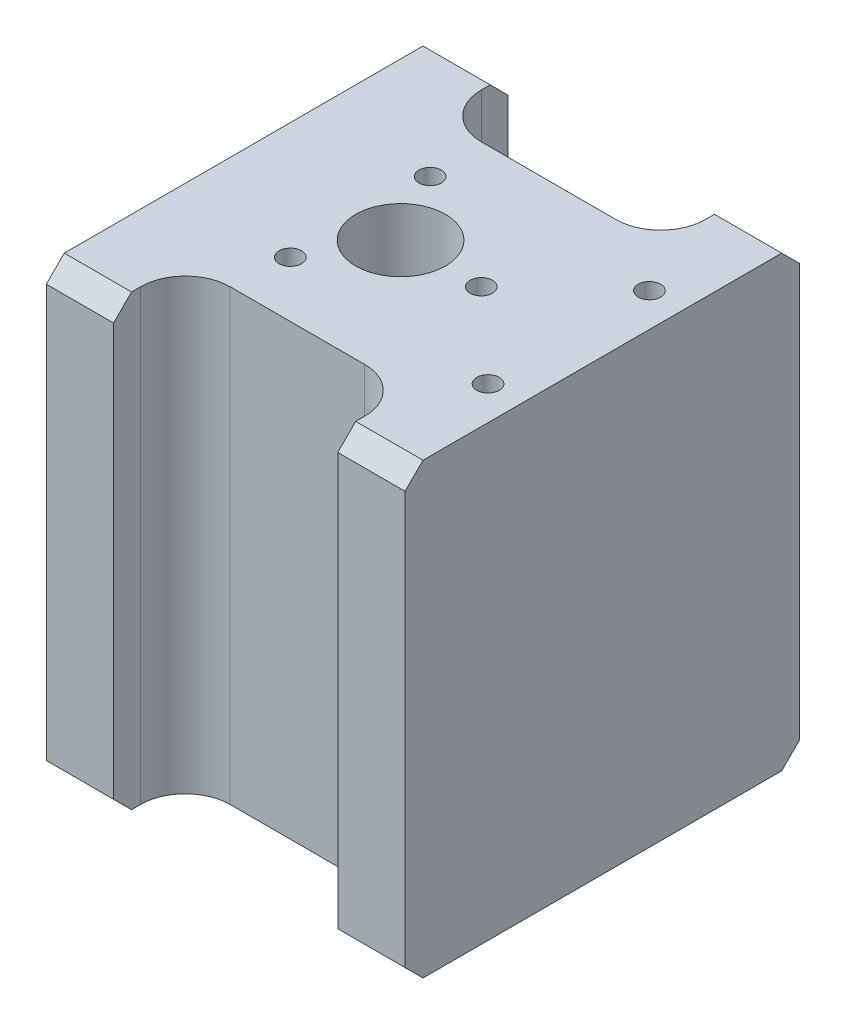
SolidWorks part; units mm, degrees
material "A6061"
ref_plane "Front Plane" through (0, 0, 0) normal (0, 0, 1) x (1, 0, 0)
ref_plane "Top Plane" through (0, 0, 0) normal (0, 1, 0) x (1, 0, 0)
ref_plane "Right Plane" through (0, 0, 0) normal (1, 0, 0) x (0, 0, -1)
sketch "Sketch1" plane through (0, 0, 0) normal (0, 0, 1) x (1, 0, 0)
  line L1 (-20, 25) -> (20, 25)
  line L2 (-20, 25) -> (-20, -25)
  line L3 (-20, -25) -> (20, -25)
  line L4 (20, 25) -> (20, -25)
  line L5 (-20, 25) -> (20, -25) construction
  line L6 (-20, -25) -> (20, 25) construction
  point P0 (0, 0)
  dimension "D1" = 40
  dimension "D2" = 50
extrude "Boss-Extrude1" add sketch "Sketch1" along normal blind 44
sketch "Sketch2" plane through (0, 25, 0) normal (0, 1, 0) x (1, 0, 0)
  line L0 (-20, -22) -> (20, -22) construction
  line L2 (-20, -44) -> (-20, 0) construction
  line L3 (20, -44) -> (20, 0) construction
  circle A0 centre (-2.5, -22) radius 5
  dimension "D1" = 10
  dimension "D2" = 17.5
extrude "Cut-Extrude1" cut sketch "Sketch2" against normal blind 20
hole_wizard "M3 Tapped Hole1" positions "Sketch4" profile "Sketch3" tap size "M3" standard "Iso"
sketch "Sketch4" plane through (0, 25, 0) normal (0, 1, 0) x (1, 0, 0)
  line L2 (2.5, -22) -> (-2.5, -22) construction
  circle A1 centre (-2.5, -22) radius 5 construction
  circle A2 centre (-2.5, -22) radius 5 construction
  point P0 (6.5, -22)
  dimension "D1" = 9
sketch "Sketch3" plane through (6.5, 25, 22) normal (1, 0, 0) x (0, 0, 1)
  line L0 (0, 0) -> (0, 8.2511)
  line L1 (0, 8.2511) -> (1.25, 7.5)
  line L2 (1.25, 7.5) -> (1.25, 0)
  line L5 (1.25, 0) -> (0, 0)
  line L10 (0, 8.2511) -> (-1.25, 7.5) construction
  line L11 (0, -6.35) -> (0, 107.95) construction
  dimension "螺纹孔钻头直径" = 2.5
  dimension "螺纹孔钻头深度" = 7.5
  dimension "导头角度" = 118
cosmetic thread "Hole thread1" parameters "D1"=6, "D2"=3
pattern_circular "CirPattern1" count 3 over 360 about axis through (-2.5, 0, 22) along (0, 1, 0) of "M3 Tapped Hole1"
hole_wizard "M4 Tapped Hole1" positions "Sketch6" profile "Sketch5" tap size "M4" standard "Iso"
sketch "Sketch6" plane through (0, -25, 0) normal (0, -1, 0) x (-1, 0, 0)
  line L0 (-20, -22) -> (20, -22) construction
  line L1 (-20, -44) -> (-20, 0) construction
  line L2 (20, -44) -> (20, 0) construction
  point P0 (-14, -32)
  point P3 (2, -32)
  point P6 (-14, -12)
  point P8 (2, -12)
  dimension "D1" = 16
  dimension "D2" = 6
  dimension "D3" = 20
sketch "Sketch5" plane through (14, -25, 32) normal (1, 0, 0) x (0, 0, -1)
  line L0 (0, 0) -> (0, 11.0914)
  line L1 (0, 11.0914) -> (1.65, 10.1)
  line L2 (1.65, 10.1) -> (1.65, 0)
  line L5 (1.65, 0) -> (0, 0)
  line L10 (0, 11.0914) -> (-1.65, 10.1) construction
  line L11 (0, -6.35) -> (0, 107.95) construction
  dimension "螺纹孔钻头直径" = 3.3
  dimension "螺纹孔钻头深度" = 10.1
  dimension "导头角度" = 118
cosmetic thread "Hole thread2" parameters "D1"=8, "D2"=4
cosmetic thread "Hole thread3" parameters "D1"=8, "D2"=4
cosmetic thread "Hole thread4" parameters "D1"=8, "D2"=4
cosmetic thread "Hole thread5" parameters "D1"=8, "D2"=4
sketch "Sketch7" plane through (0, -25, 0) normal (0, -1, 0) x (1, 0, 0)
  line L0 (-20, 44) -> (20, 44) construction
  line L1 (12.5, 44) -> (-12.5, 44)
  line L2 (12.5, 44) -> (12.5, 36)
  line L3 (12.5, 36) -> (-12.5, 36)
  line L4 (-12.5, 44) -> (-12.5, 36)
  line L5 (0, 0) -> (0, 44) construction
  line L6 (-20, 22) -> (20, 22) construction
  line L7 (-20, 44) -> (-20, 0) construction
  line L8 (20, 44) -> (20, 0) construction
  line L9 (12.5, 8) -> (-12.5, 8)
  line L10 (12.5, 0) -> (12.5, 8)
  line L11 (12.5, 0) -> (-12.5, 0)
  line L12 (-12.5, 0) -> (-12.5, 8)
  dimension "D1" = 25
  dimension "D2" = 8
extrude "Cut-Extrude2" cut sketch "Sketch7" against normal through all
chamfer "Chamfer1" distance 2 angle 45 8 edges at (-16.25, 25, 0) (-16.25, 25, 44) (-16.25, -25, 44) (-16.25, -25, 0) (16.25, -25, 0) (16.25, -25, 44) (16.25, 25, 44) (16.25, 25, 0)
fillet "Fillet1" radius 5 4 edges at (-12.5, 0, 36) (12.5, 0, 36) (-12.5, 0, 8) (12.5, 0, 8)
hole_wizard "M3 Tapped Hole2" positions "Sketch9" profile "Sketch8" tap size "M3" standard "GB"
sketch "Sketch9" plane through (0, 25, 0) normal (0, 1, 0) x (1, 0, 0)
  line L0 (-2.5, -22) -> (29.898, -22) construction
  line L3 (16.25, -44) -> (16.25, -32.2693) construction
  line L4 (20, -44) -> (12.5, -44) construction
  point P0 (16.25, -31)
  point P2 (16.25, -13)
  dimension "D1" = 18
sketch "Sketch8" plane through (16.25, 25, 31) normal (1, 0, 0) x (0, 0, 1)
  line L0 (0, 0) -> (0, 9.2511)
  line L1 (0, 9.2511) -> (1.25, 8.5)
  line L2 (1.25, 8.5) -> (1.25, 0)
  line L5 (1.25, 0) -> (0, 0)
  line L10 (0, 9.2511) -> (-1.25, 8.5) construction
  line L11 (0, -6.35) -> (0, 107.95) construction
  dimension "螺纹孔钻头直径" = 2.5
  dimension "螺纹孔钻头深度" = 8.5
  dimension "导头角度" = 118
cosmetic thread "Hole thread6" parameters "D1"=6, "D2"=3
cosmetic thread "Hole thread7" parameters "D1"=6, "D2"=3
